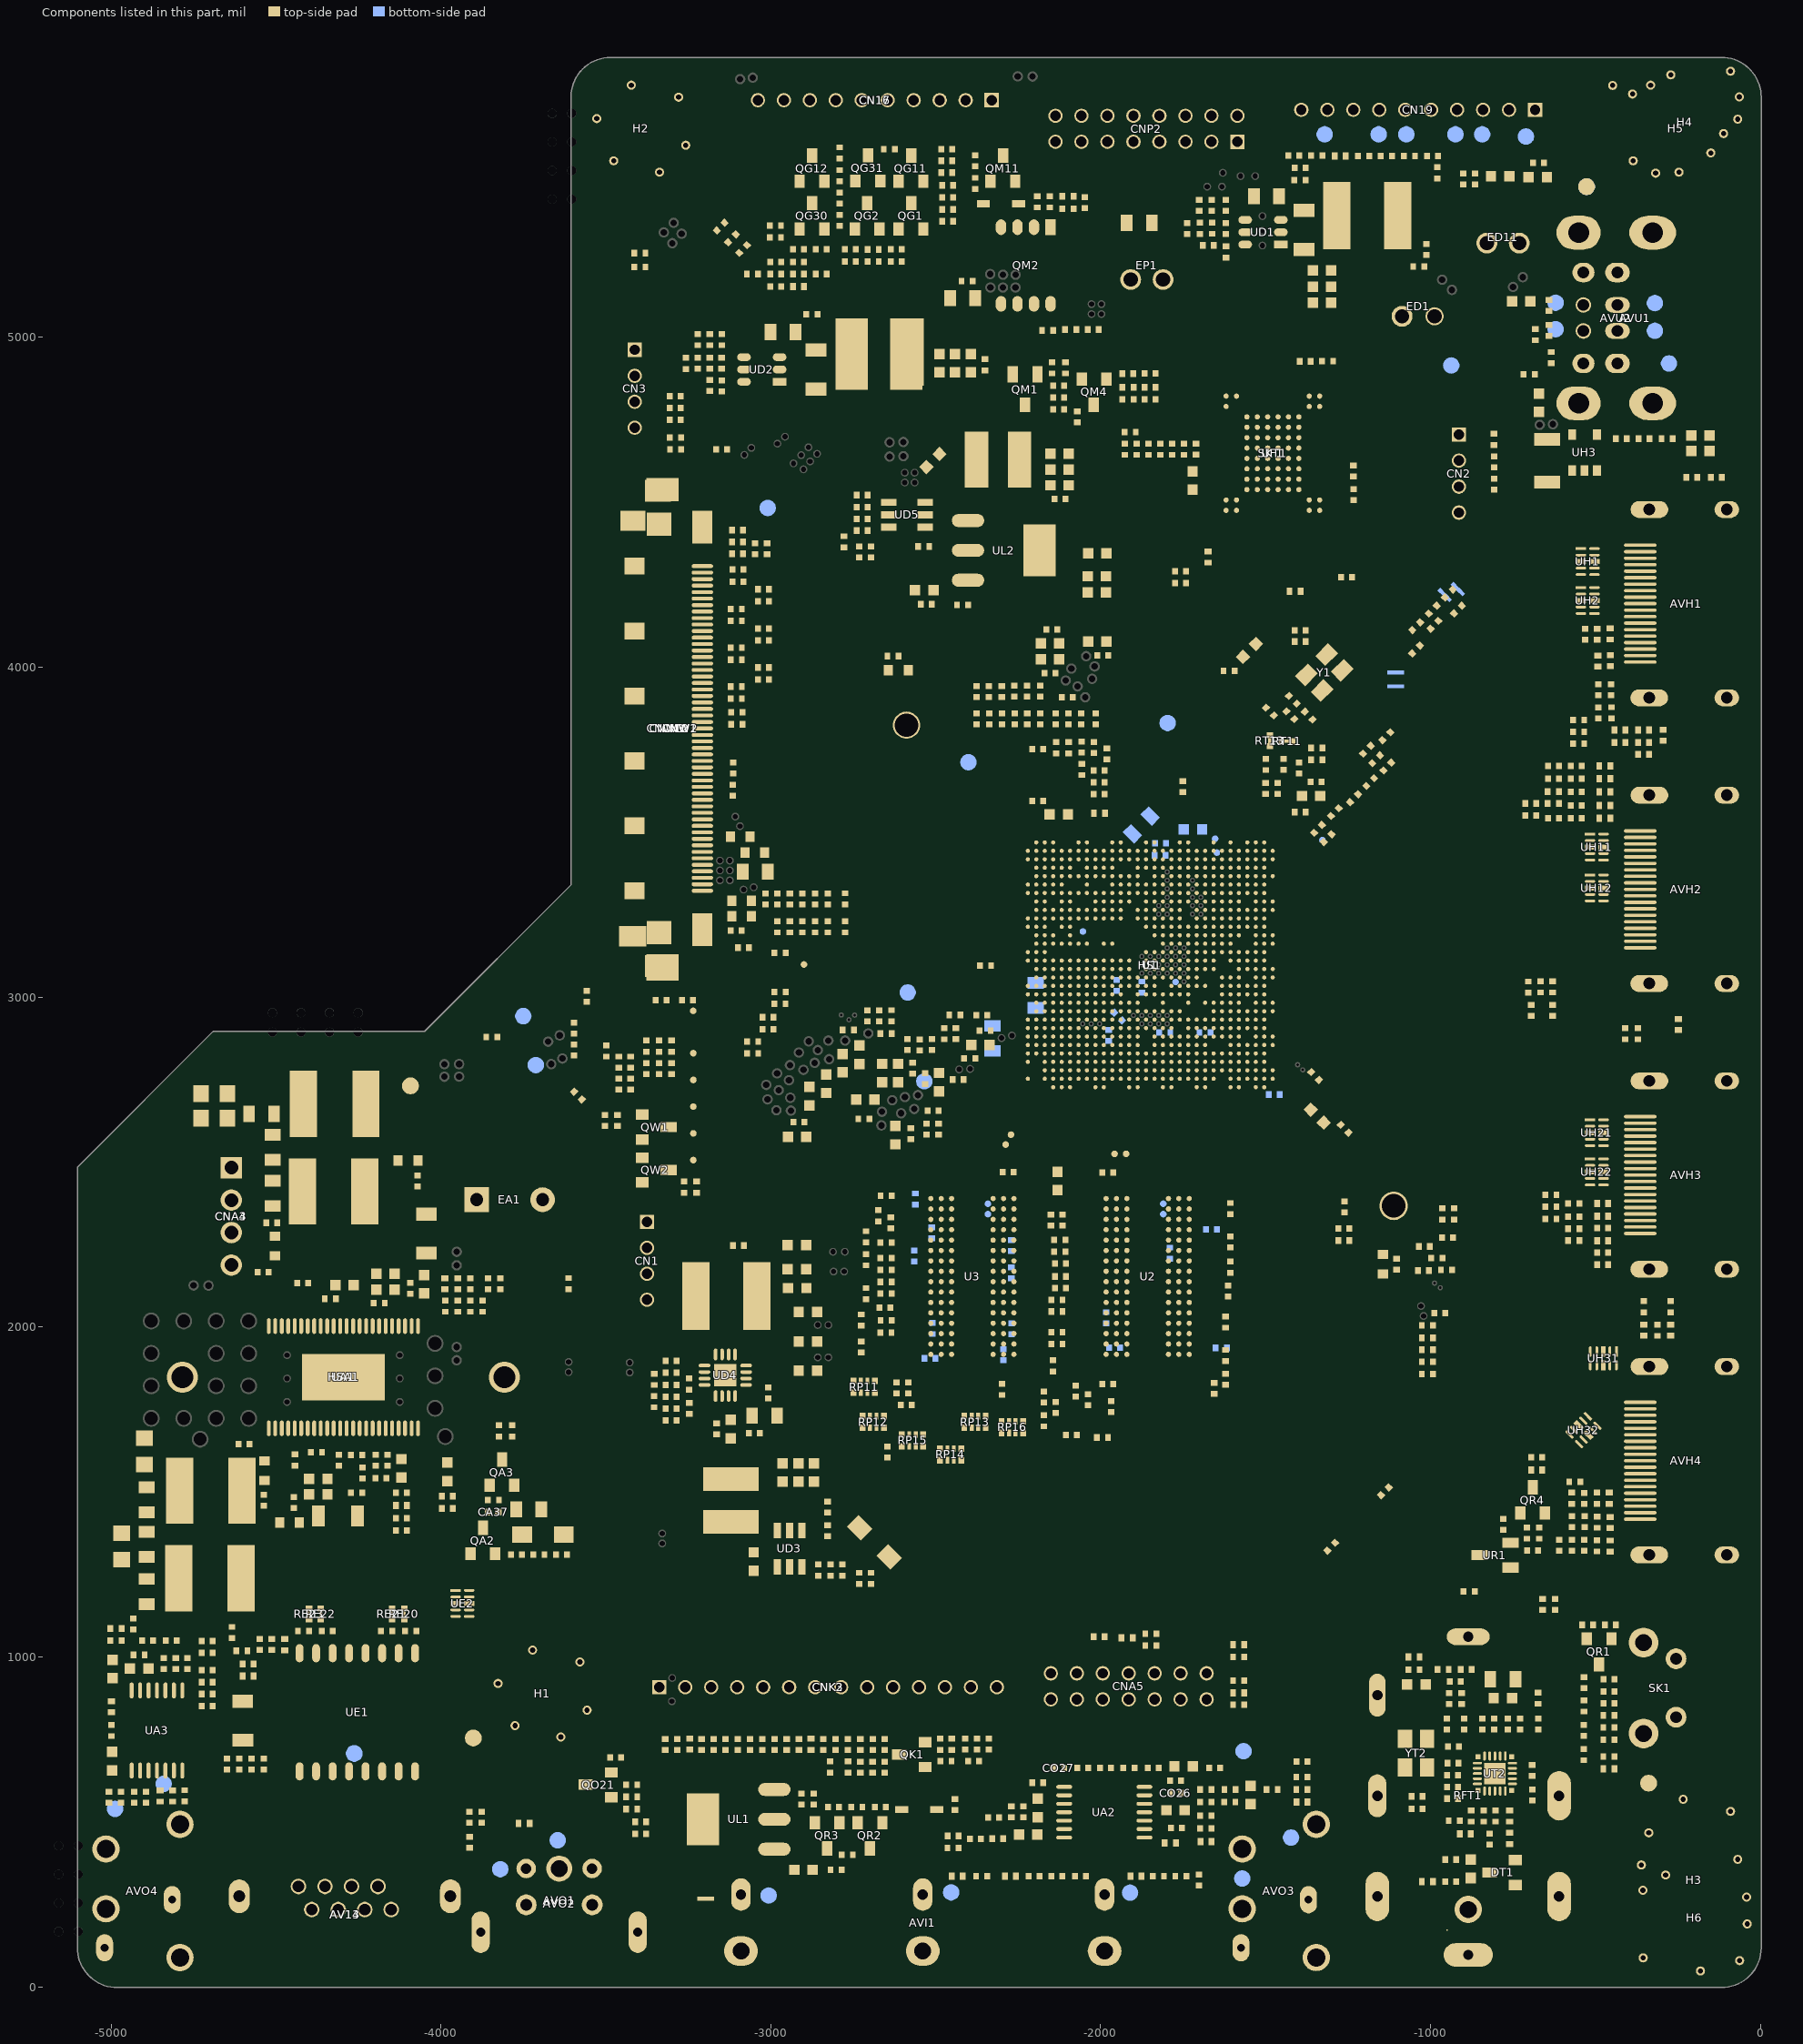
[diagram p0: the components of this part, seen from the top]
# Altium PCB MISC86290.PcbDoc (part 30 of 31)
Units mil, origin at the board's own origin, x right, y up, seen from the top; angles counter-clockwise.
Board outline 5104.71 x 5851.49 mil, 2 copper layers (TopLayer, BottomLayer), stack 61.855 mil thick; 1026 components, 667 nets, 4280 pads, 2294 vias.

## Other copper (continued)
BottomLayer:
  rectangle net GND: -1714.23,3506 -1676.5,3598.5
  rectangle net GND: -1723.5,2865.75 -1684.5,2918.16
  rectangle net GND: -3929.45,78 -3834,254.33
  rectangle net GND: -3978,211 -3889,336.95
  rectangle net GND: -4668,205 -4612.21,335.6
  rectangle: 1509.88,1166.59 1640.08,1245.33
  rectangle net GND: -644,5205 -158,5383.07
  rectangle net GND: -999.5,45.5 -767.5,160
  rectangle net GND: -1236.5,176.5 -1095.5,377
  rectangle net GND: -685,476 -533,705.5
  rectangle net GND: -1723.5,2918.16 -1658.13,2982
  rectangle net GND: -369.5,5302.5 -225,5406
  region net AVDD_EAR33/AU33: -1379.69,2771.69 -1370.69,2771.69 -1354.1,2755.1 -1354.1,2741.08 -1365.08,2741.08 -1372.94,2748.94 -1372.94,2764.94
  pour cut-out: -2568.5,693.5 -2536.5,693.5 -2529,701 -2521,701 -2521,683 -2504.5,666.5 -2533.6,637.4 -2546.39,637.4
  pour cut-out: -3287.55,3022.65 -3287.55,2990.74 -3270.17,2973.36 -3287,2956.53 -3287,2849 -3416,2849 -3418.88,2846.12 -3418.88,2983.69 -3387.76,3014.8
  pour cut-out: -952.79,1738.01 -1001.99,1738.01 -1001.66,1738.34 -1001.66,1760.19 -985.35,1776.5 -961.32,1776.5
  pour cut-out: -3092,3573.24 -3131.74,3573.24 -3146.5,3588 -3154,3580.5 -3159.5,3580.5 -3159.5,3538.5 -3128.14,3507.14 -3120,3507.14
  region net 3V3_M: -2004.5,3945 -2031,3945 -2060,3974 -2060,4044 -2054.5,4049.5 -2017.5,4049.5 -2001.5,4033.5 -2001.5,3992.5 -1985,3976 -1985,3965
  pour cut-out: -4598.5,226 -4598.5,185 -4593.5,180 -4551.5,180 -4549,182.5 -4549,239.5 -4550.5,241 -4584,241 -4597.5,227.5
  pour cut-out: -1678.84,1557.5 -1687.65,1566.3 -1687.65,1573 -1672.35,1573 -1670.34,1571 -1672.84,1568.5 -1672.84,1556.64
  region net NetCN2_4: 213 vertices and 0 holes, not listed, extent -934.4,4394.99 -893.6,4468.89
  region: -4442,180.67 -4442,62.56 -4134,62.56 -4134,180.67
  pour cut-out: -294.25,5156.5 -258.25,5120.5 -258.25,4895.5 -288.25,4865.5 -438.25,4865.5 -470.25,4897.5 -470.25,5119.5 -433.25,5156.5
  region net VCC_PANEL: -2376.26,5172.74 -2338.26,5210.74 -2253.26,5210.74 -2240.26,5197.74 -2240.26,5142.74 -2299.26,5083.74 -2376.26,5083.74
  region net 5V_M: -681,4778 -689,4770 -689,4721 -680,4712 -621,4712 -611.74,4721.26 -611.74,4741.74 -648,4778
  region net 3V3_M: -1759.52,3323.09 -1759.52,3264.26 -1738.02,3242.76 -1692.2,3242.76 -1687.02,3247.94 -1687.02,3279.26 -1691.23,3279.26 -1722.02,3310.05
  region net 5V_M: -3621,1911 -3459,1911 -3410.5,1862.5 -3421,1852 -3619,1852 -3625,1858 -3625,1907
  region net 0.95V_VDDC: -2759,2888 -2896,2888 -3053,2731 -3053,2710 -3039,2696 -2877,2696 -2761.25,2811.75 -2761.25,2883.53 -2757.93,2886.84
  region net 0.95V_VDDC: -3053,2731 -3053,2695 -2977,2619 -2921,2619 -2836,2704 -2836,2788 -2996,2788
  region net 5V_M: -3461,1911 -3422.5,1911 -3410.5,1899 -3410.5,1862 -3420.5,1852 -3456.5,1852 -3467.5,1863 -3467.5,1904.5
  pour cut-out: -1775.16,2878.47 -1836.34,2878.47 -1836.34,2878.46 -1836.34,2890.97 -1834,2893.31 -1775.16,2893.31
  region net GND: -2501.72,1910.03 -2469.72,1910.03 -2469.72,1854.03 -2485.72,1838.03 -2501.72,1838.03 -2501.72,1910.03
  region net GND: -2061.72,2046.03 -2061.72,2078.03 -1973.72,2078.03 -1973.72,2046.03 -2061.72,2046.03
  region net GND: -2341.72,1874.03 -2341.72,1906.03 -2253.72,1906.03 -2253.72,1874.03 -2341.72,1874.03
  region net GND: -2545.72,1954.03 -2545.72,1986.03 -2457.72,1986.03 -2457.72,1954.03 -2545.72,1954.03
  region net GND: -1905.72,1922.03 -1945.72,1922.03 -1945.72,1998.03 -1905.72,1998.03 -1905.72,1922.03
  region net GND: -2313.72,2206.03 -2313.72,2238.03 -2225.72,2238.03 -2225.72,2206.03 -2313.72,2206.03
  region net GND: -1601.72,1898.03 -1621.72,1898.03 -1621.72,1974.03 -1601.72,1974.03 -1601.72,1898.03
  region net GND: -1613.72,2262.03 -1653.72,2262.03 -1653.72,2338.03 -1613.72,2338.03 -1613.72,2262.03
  region net GND: -2581.72,2170.03 -2581.72,2202.03 -2525.72,2202.03 -2509.72,2186.03 -2509.72,2170.03 -2581.72,2170.03
  region net 1V5_DDR: -2476,2787 -2560.25,2787 -2654,2693.25 -2654,2677 -2647,2670 -2621,2670 -2607,2684 -2547,2684 -2476,2755
  region net LINEOUT_LL: -5024.75,458.5 -4945,458.5 -4940,453.5 -4940,380.5 -4944,376.5 -5023,376.5 -5033,386.5 -5033,450.25
  region net LINEOUT_LL: -5024.75,277.4 -4945,277.4 -4940,272.4 -4940,199.4 -4944,195.4 -5023,195.4 -5033,205.4 -5033,269.15
  region net GND: -5020,159 -4951,159 -4947,155 -4947,81 -4951,77 -5017,77 -5026,86 -5026,153
  pour cut-out: -5106,522 -4951.93,522 -4936.93,507 -4936.93,466.57 -4945,458.5 -5114.5,458.5 -5128,472 -5128,500
  pour cut-out: -4928,389 -4941,402 -5033,402 -5105,330 -5105,172.65 -5099.68,167.32 -4954.77,167.32 -4928,194.09
  pour cut-out: -3984,228 -3984,190 -3992,182 -4025,182 -4041,198 -4041,229 -4032,238 -3994,238
  pour cut-out: -516,5184 -381.61,5184 -368.01,5170.4 -368.01,5167.99 -376,5160 -525,5160 -525,5175
  region net CNW12_PIN42: -3117,3561 -3120,3558 -3120,3456.29 -3090,3426.29 -3090,3340.5 -3097,3333.5 -3097,3320.5 -3089,3312.5 -3049.5,3312.5 -3039,3323 -3039,3433.5 -3075,3469.5 -3075,3544 -3092,3561
  region net NetCN3_4: 213 vertices and 0 holes, not listed, extent -3432.9,4652.5 -3392.1,4726.39
  region net NetCN1_4: 213 vertices and 0 holes, not listed, extent -3395.65,2008.62 -3354.85,2082.52
  region net GND: -950.5,1113 -829,1113 -797.5,1081.5 -797.5,1034.5 -823,1009 -963,1009 -990,1036 -990,1110 -979.5,1120.5
  region net GND: -1178.5,674.5 -1127.5,674.5 -1103.5,650.5 -1103.5,505 -1120.5,488 -1189,488 -1227.5,526.5 -1227.5,631 -1197,661.5 -1197,679
  region net GND: -591.5,372 -638.5,372 -668.5,342 -668.5,211.5 -633,176 -599.5,176 -574,201.5 -574,231 -562.5,242.5 -562.5,372 -577.5,387
  region net GND: -1169,782 -1208,821 -1208,958 -1193,973 -1125,973 -1105,953 -1105,844 -1154,795 -1161.5,795 -1163,793.5
  region net GND: -1855.16,3030.54 -1969.76,3030.54 -1980.54,3019.77 -1979.36,3019.77 -1942.09,2982.5 -1863.57,2982.5 -1847.07,2999 -1815.5,2999
  region net GND: -1870.5,3437 -1870.5,3461.72 -1944.28,3535.5 -1963.61,3535.5 -1976,3523.11 -1976,3495 -1908,3427 -1867.5,3427
  pour cut-out: -3171.5,4711.5 -3171.5,4721.18 -3242.09,4791.77 -3429.05,4791.77 -3442.41,4805.13 -3442.41,4705.26 -3394.64,4657.5 -3356,4657.5
  pour cut-out: -3223.25,4579.25 -3223.25,4637.28 -3193.73,4666.8 -3207,4680.07 -3207,4689.5 -3304,4689.5 -3337.84,4655.66 -3337.84,4626.98
  region net GND: -285.8,4867.95 -288.25,4865.5 -576.77,4865.5 -613.77,4902.5 -624,4902.5 -609,4887.5 -609,4850.98 -618.84,4841.15 -597,4819.31 -597,4745.42 -597.39,4745.03 -588.5,4736.14 -588.5,4730 -546.5,4730 -542.5,4726 -500,4726 -453,4773 -425,4773 -354.5,4702.5 -226.5,4702.5 -184,4745 -184,4863 -165.5,4881.5
  pour cut-out: -578.5,4888 -668,4977.5 -668,5127 -649,5146 -623,5146 -596,5173 -562,5173 -502.5,5113.5 -502.5,5027
  region net GND: -3369,942.5 -3373,946.5 -3396,946.5 -3400.5,951 -3400.5,952 -3384,952 -3373,963 -3369,963
  pour cut-out: -3492,638.5 -3380,638.5 -3359.5,618 -3338,639.5 -3318,639.5 -3318,683.62 -3346.87,654.75 -3486,654.75
  region net 1V5_DDR: -2537.5,2697 -2537.5,2657 -2602,2592.5 -2680,2592.5 -2686.5,2599 -2686.5,2660.75 -2590.75,2756.5 -2525,2756.5 -2522.5,2759
  region net 3V3_STB: -1428.16,2740.51 -1225.5,2537.85 -1225.5,2476.54 -1428.91,2679.95 -1428.91,2740.51
  region net GND: -1610.5,2899 -1539.34,2899 -1530.32,2889.98 -1611.22,2889.98 -1616.84,2895.6 -1616.84,2896.14
  region net 0.95V_VDDC: -2014.5,3136 -2041,3109.5 -2358.5,3109.5 -2375.5,3092.5 -2375.5,3041 -2354,3019.5 -1993.5,3019.5 -1971.5,3041.5 -1971.5,3136
  region net 3V3_STB: -1666.96,2902.49 -1638.89,2902.49 -1620.18,2883.78 -1533.19,2883.78 -1518.51,2869.1 -1518.51,2859.11 -1522.42,2855.2 -1567.1,2855.2 -1579.1,2867.2 -1628.52,2867.2 -1644.02,2882.7 -1658.94,2882.7 -1667.19,2890.95 -1667.19,2901.92
  region net GND: -1389,2747.81 -1389,2760.81 -1427.9,2799.71 -1427.9,2801.7 -1524.73,2898.53 -1536.16,2898.53 -1536.16,2897.34 -1406.32,2767.5 -1406.32,2753.9 -1398.15,2745.73 -1396.91,2745.73
  pour cut-out: -702.64,3166.16 -702.64,3161.48 ccw(c-682.52,3161.48) -696.75,3147.25 ccw(c-681,3163) -681,3140.73 -570.9,3140.73 ccw(c-570.9,3151.9) -563,3144 cw(c-535.62,3171.38) -574.34,3171.38 -574.34,3197 cw(c-574.34,3233.59) -600.22,3207.72 -612.5,3220 ccw(c-636.26,3196.24) -636.26,3229.84 -666.84,3229.84
  text ".GBL" at 2085.1,1188.26 h60
  text "BottomLayer" at 1662.68,1186.76 h60

## Silkscreen, mask and mechanical layers (free items; w line width, h text height)
TopOverlay:
  drawing of 267 lines, arcs and shapes, not listed
  text "Solder Mask:" at 1375,6344.9 h60
  text "IPC SM-840" at 1787.5,6343.9 h60
  text "Silkscreen Color:" at 2553.5,6343.9 h60
  text "White" at 3032.5,6343.9 h60
  text "Units:" at 2553.5,6244.9 h60
  text "PTH Copper Thickness:" at 1375,6243.9 h60
  text ">20um" at 2048.5,6242.9 h60
  text "mm" at 2751.5,6243.4 h60
  text "Dielectric Constant Er@1GHz To 1MHz:" at 1374.66,6144.92 h60
  text "4.2 --- 4.6" at 2554.16,6145.42 h60
  text "Panel Size:" at 1373,6046.4 h60
  text "2L,2,111.28×148.50mm,FR4(TG150-CTI175),1OZ,Green,OSP,1.2mm" at 1678.16,6046.42 h60
  text "Silkscreen on PTH:" at 1373.5,5944.9 h60
  text "Primary Side Retained;" at 1891.5,5943.9 h60
  text "Secondary Side  Removed for Soldering" at 2553.5,5942.4 h60
  text "Special Requirements" at 1372.49,5854.21 h60
  text "For engineering questions with no reply within 2 hours, call: PHONE_A" at 3259.16,5846.92 h60
  text "POWER" at -2125,5789.5 h60
  text "EXT-WIFI" at -1017,5788 h60
  text "2" at -6473.13,5777.09 h160 r180
  text "1. Lead-free HASL (HAL_LF, Lead Free Hot Air Leveling)" at 1963.38,5750.63 h60
  text "2. Organic solderability preservative (OSP, Organic Solderability Preservatives)" at 1963.38,5666.63 h60
  text "3. Electroless nickel immersion gold (ENIG, Electroless Nickel/Immersion Gold)" at 1961.88,5575.13 h60
  text "Plated Technics" at 1447.5,5540.4 h60
  text "4. Electroless nickel immersion gold + gold finger (ENIG_G/F, Electroless Nickel/Immersion Gold + Gold Finger)" at 1963.38,5494.63 h60
  text "5. Gold plating (Gold_plated, Gold-plated)" at 1964.38,5414.13 h60
  text "LOCAL DIMMING" at -3148,5389 h60 r90
  text "6. Gold plating + gold finger (Gold_Plated_G/F, Gold-plated + Gold Finger)" at 1964.88,5336.13 h60
  text "PM-UART" at -3565,5118.5 h60
  text "Impedance Control" at 1377.24,5107.54 h60
  text "Target Impedance" at 2174.07,5107.64 h60
  text "Width & Clearance" at 2919.9,5107.41 h60
  text "Layer(s)" at 3688.21,5107.72 h60
  text "75 +/- 10% Ohm" at 2196.27,5006.94 h60
  text "G/12/15.8/12/G mil" at 2877.32,5006.26 h60
  text "layer 1" at 3688.21,5006.38 h60
  text "Single End Impedance" at 1377.24,4960.72 h60
  text "DEBUG" at -1025,4865 h60
  text "[ Zo ]" at 1600.74,4823.47 h60
  text "G/5/7/5/7/5/G mil" at 2887.32,4615.26 h60
  text "100 +/- 10% Ohm" at 2183.27,4614.25 h60
  text "layer 1" at 3704.5,4612.5 h60
  text "Differential Impedance" at 1377.1,4559.14 h60
  text "[ Zo ]" at 1600.23,4435.8 h60
  text "( G: Ground )" at 1510.31,4328.3 h60
  text "90 +/- 10% Ohm" at 2209.32,4316.26 h60
  text "G/5/11/5/11/5/G mil" at 2887.32,4312.76 h60
  text "layer 1&2" at 3703.5,4307.5 h60
  text "Common Mode Impedance" at 1356.87,4106.62 h60
  text "[ Zc ]" at 1604.87,4025.62 h60
  text "Refer to Gerber documents GTP&GBP for Stencil aperture design" at 2271.93,3761.43 h60
  text "[Bottom-side parts: stencil per BOM]" at 2271.2,3674.01 h60
  text "Stencil" at 1371.16,3664.42 h60
  text "New" at 2269.83,3566.88 h60
  text "V_by_one" at -3017,3549 h60 r90
  text "Test fixture (Testing jig)" at 1369.25,3468.78 h60
  text "The same as XXXXXXXXXXX XXXXXX" at 2258,3468.5 h60
  text "The same as XXXXXXXXXXX XXXXXX" at 2258.5,3375.5 h60
  text "Wave-soldering fixture (Wave-soldering jig)" at 1371.47,3370.54 h60
  text "Solder paste" at 2269.45,3268.76 h60
  text "Production process" at 1369.95,3267.26 h60
  text "[Process and notes]" at 1550.16,3182.42 h60
  text "Back-side panelization" at 2267.22,3069.97 h60
  text "Special requirements (Special Requirements)" at 1370.95,3069.26 h60
  text "Chip parts on solder side taller than 2mm (wave soldering)" at 1370.66,2967.92 h60
  text "Packaging notes (Package Attention)" at 1370.33,2871.71 h60
  text "[Easily damaged parts]" at 1611.66,2786.92 h60
  text "New footprint matching (Footprint Matching)" at 1370.33,2671.71 h60
  text "[New component footprint]" at 1597.66,2587.92 h60
  text "(Automated Testing Support)" at 1688.66,2473.42 h45
  text "Automatic test support" at 1370.16,2469.92 h60
  text "[Reserved vacuum nozzle and press-pin positions]" at 1530.66,2385.42 h60
  text "Layer Stack Up Detail for" at 1511.26,2025.89 h100
  text ".Pcb_File_Name_No_Path" at 2572.08,2025.89 h100
  text "FRC PLACE HOLDER" at -3520.75,1975 h60 r90
  text "Layer" at 1675.62,1878.17 h50
  text "Gerber" at 2047.34,1878.17 h50
  text "Layer" at 2358.49,1878.17 h50
  text "Layer" at 2994.72,1878.17 h50
  text "Copper" at 3783.63,1878.17 h50
  text "Dielectric" at 4095.41,1878.17 h50
  text "Height" at 4095.5,1833 h50
  text "Stack up" at 2992,1832 h50
  text "Name" at 1675.62,1825.79 h50
  text "Document" at 2047.34,1825.79 h50
  text "Ordor" at 2358.49,1825.79 h50
  text "Thickness" at 3783.63,1825.79 h50
  text "SPEAKER" at -4982,1714 h60 r90
  text "TopOverlay" at 1675.33,1592.93 h60
  text ".GTO" at 2084.9,1590.37 h60
  text "0.4mil" at 4092.72,1505.34 h60
  text "1" at 2411.69,1402.19 h60
  text "1.4mil" at 3796.68,1402.13 h60
  text "2" at 2411.74,1189.15 h60
  text "1.4mil" at 3794.97,1188.14 h60
  text "ATMOS AND DEBUG" at -2166,1146 h60
  text "0.4mil" at 4095.4,1093.46 h60
  text "Notes:" at 1347.19,530.59 h80
  text "1. No Plated Through Hole  overlap each other should be combined ,Residues between them should be eliminated." at 1346.32,442.68 h60
  text "2. Plated Through Hole superposition should be made as a bigger one." at 1346.26,366.58 h60
  text "3. When there is not enough space for UL authentication marking,Manufacturer ID code and the Bar Code frame," at 1346.32,298.08 h60
  text "only the Manufacturer  ID code is needed and layed wherever it can be." at 1404.7,227.39 h60
  text "4. Spacing between two pads of IC package should be covered with solder oil." at 1346.32,150.62 h60
  text "5. All trace should be covered with green oil unless otherwise specified. If discovers unusually, please confirm with us." at 1346.32,77.21 h60
  text "1" at -2289.22,69.37 h160
  text "6. Silkscreen overlaped SMD pads should be removed directly." at 1346.32,3.9 h60
  text "7. The width of Carbon Sprayed must be 16mil wider than its trace." at 1346.32,-67.14 h60
  text "8. Bridging Thickness of V-cut  should be kept within 0.3±0.1mm when the width of single piece bare board is smaller than 20mm." at 1346.32,-141.57 h60
  text "9. There is no need to plugged with green oil when the diameter of vias is bigger than 0.6mm." at 1346.32,-223.4 h60
  text "10. All vias under BGA must be covered and plugged with Solder oil." at 1346.33,-303.27 h60
BottomOverlay:
  rectangle: 1509.88,974.82 1640.08,1053.56
  region: -400,2670 -400,2694.1 -425.9,2720 -485,2720 -500,2705 -500,2215 -443,2215 -443,2627
  region: -435,3160 -493,3160 -493,3520 -435,3520
  region: -440,3315 -440,3275 -420,3255 -420,3213.5 -437.25,3196.25 -450,3209 -450,3305
  region: 16 vertices and 3 holes, not listed, extent -3400.9,113.96 -3115.45,536.16
  lines w5: -4669,2530 -4867,2530 -4867,2143 -4665,2143 ; -3441.5,4690 -3565.5,4690 -3565.5,4996 -3435.5,4996 ; -3399,2355 -3644,2355 -3644,2046 -3398,2046 ; -3385,912 -3385,1107.61 -2264,1107.61 -2264,907.34 ; -2193,975.73 -2193,1297 -1632,1297 -1632,967 ; -1534,5549 -1505,5520 -1501,5520 -1343,5520 -1343,5475 ; -1430,5710 -1430,5832 -646,5832 -646,5717 ; -1359,5491 -1343,5475 ; -1327,5491 -1343,5475 ; -933,4433 -1102,4433 -1102,4743 -933,4743 ; 2060.78,974.82 2060.78,1053.56 ; -1365.48,5202.5 -926,5202.5 -926,5475 -1335,5475 -1365.48,5475 -1365.48,5202.5 ; -1206.92,1240.13 -773.85,1240.13 -773.85,1692.89 -1206.92,1692.89 -1206.92,1240.13 ; 1509.88,974.82 2241.92,974.82 2241.92,1053.56 1509.88,1053.56 1509.88,974.82
  text "MISO" at -2429.5,5806.5 h50
  text "EN" at -2307,5806 h50
  text "GND" at -2920,5805 h50
  text "HSY" at -2764,5805 h50
  text "GND" at -2591.5,5805.5 h50
  text "GND" at -1307,5785 h60
  text "GND" at -1167,5784 h60
  text "3V3" at -723,5784.5 h60
  text "WAKE" at -986,5783 h60
  text "DP" at -884,5782 h60
  text "LD" at -2855.5,5767.5 h50
  text "CLK" at -2514.5,5767 h50
  text "CSN" at -2965,5766 h50
  text "CSZ" at -2356,5766.5 h50
  text "VSY" at -2681.5,5765.5 h50
  text "REG" at -1112,5737 h60
  text "GND" at -941,5737 h60
  text "DM" at -811,5737 h60
  text "3V3" at -657.5,5737.5 h60
  text "HOST" at -1241,5736 h60
  text "12V" at -1103,5371 h50 r270
  text "GND" at -1063,5371 h50 r270
  text "12V" at -1147,5370 h50 r270
  text "VCC" at -1021,5370 h50 r270
  text "ADJ" at -1321,5369 h50 r270
  text "DIM" at -1278,5369 h50 r270
  text "GND" at -1234,5369 h50 r270
  text "GND" at -1191,5369 h50 r270
  text "GND" at -1191,5264 h50 r270
  text "GND" at -1233,5263 h50 r270
  text "12V" at -1147,5263 h50 r270
  text "GND" at -1063,5263 h50 r270
  text "BLO" at -1319,5262 h50 r270
  text "PWN" at -1277,5262 h50 r270
  text "12V" at -1102,5262 h50 r270
  text "VCC" at -1020,5261 h50 r270
  text "POWER&INVERTER" at -934,5213 h50
  text "USB IN" at -66.15,4947.64 h60 r270
  text "3V3" at -3464.25,4940.75 h50
  text "GND" at -3460,4864.5 h50
  text "RX2" at -3464.25,4783.27 h50
  text "TX2" at -3464.25,4704.53 h50
  text "3V3" at -968,4684.28 h60
  text "GND" at -971,4594.68 h60
  text "HDMI 4(2.0) (ARC)IN" at -46,4545 h60
  text "SCL" at -978,4517.68 h60
  text "SDA" at -975.5,4446.5 h60
  text "HDMI 3 IN(2.0)" at -555,3150 h60 r270
  text "HDMI 2 IN(2.0)" at -38,2828 h60
  text "ROUT+" at -4703,2473 h50
  text "ROUT-" at -4703,2373 h50
  text "TX1" at -3424,2300.74 h60
  text "LOUT-" at -4703,2278 h50
  text "RESETN" at -3424,2222 h60
  text "LOUT+" at -4703,2173 h50
  text "ALIVE" at -3424,2143.26 h60
  text "RCR" at -3424,2064.52 h60
  text "HDMI 1 IN(2.0)(UART)" at -34,1947 h60
  text "SCL" at -2171,1140 h60 r270
  text "GND" at -2092.26,1140 h60 r270
  text "MUTE" at -2013.52,1140 h60 r270
  text "3V3" at -1934.78,1140 h60 r270
  text "SD1" at -1856.04,1140 h60 r270
  text "SD" at -1777.3,1140 h60 r270
  text "MCK" at -1698.56,1140 h60 r270
  text "SDA" at -2171,1013 h60 r270
  text "GND" at -2092.26,1013 h60 r270
  text "RST" at -2013.52,1013 h60 r270
  text "3V3" at -1934.78,1013 h60 r270
  text "SD2" at -1856.04,1013 h60 r270
  text "WS" at -1777.3,1013 h60 r270
  text "BCK" at -1698.56,1013 h60 r270
  text ".GBO" at 2085.51,997.85 h60
  text "BottomOverlay" at 1663.84,996.86 h60
  text "Reset" at -77,899 h60
  text "RF IN" at -673,186 h60
  text "LINE OUT" at -4912,62.5 h60 r270
  text "COAX OUT" at -3493,58 h60
  text "AV INT" at -2274,30 h60
  text "RJ45 IN" at -4201,16 h60
  text "HEADPHONE OUT" at -1400,14 h60
  text "OPTICAL OUT" at -3453,12 h60
TopPaste:
  rectangle: 1509.88,1668.23 1640.08,1746.97
  lines w5: 2060.78,1668.23 2060.78,1746.97 ; 1509.88,1668.23 1509.88,1746.97 2241.92,1746.97 2241.92,1668.23 1509.88,1668.23
  text "TopPaste" at 1675.33,1689.46 h60
  text ".GTP" at 2084.9,1687.33 h60
BottomPaste:
  rectangle: 1509.88,880.67 1640.08,959.41
  lines w5: 2060.78,880.67 2060.78,959.41 ; 1509.88,880.67 1509.88,959.41 2241.92,959.41 2241.92,880.67 1509.88,880.67
  text "BottomPaste" at 1662.68,903.65 h60
  text ".GBP" at 2085.78,898.53 h60
TopSolder:
  rectangle: 1509.88,1478.28 1640.08,1557.02
  lines w5: 2060.78,1478.28 2060.78,1557.02 ; 1509.88,1478.28 1509.88,1557.02 2241.92,1557.02 2241.92,1478.28 1509.88,1478.28
  text "TopSolder" at 1675.83,1498.38 h60
  text ".GTS" at 2084.9,1496.73 h60
BottomSolder:
  drawing of 50 lines, arcs and shapes, not listed
  text "BottomSolder" at 1662.68,1090.06 h60
  text ".GBS" at 2084.86,1089.17 h60
过炉治具:
  drawing of 232 lines, arcs and shapes, not listed
3D和装配:
  circle w2.5: c444.93,3607.26 r1.25
  circle w2.5: c1115.74,905.51 r1.25
  circle w2.5: c1273.22,1594.49 r1.25
  circle w2.5: c1430.71,2460.63 r1.25
  circle w2.5: c-885.83,-966.64 r1.25
  circle w2.5: c-1968.51,-1124.12 r1.25
  circle w2.5: c649.6,3326.77 r1.25
  circle w2.5: c649.6,4192.92 r1.25
  circle w2.5: c649.6,4192.92 r1.25
  circle w2.5: c649.6,3326.77 r1.25
  circle w2.5: c-2421.38,1730.26 r1.25
  circle w2.5: c-2421.38,1730.26 r1.25
  circle w2.5: c-2303.27,1848.37 r1.25
  circle w2.5: c-2303.27,1848.37 r1.25
  circle w2.5: c-2303.27,1848.37 r1.25
  circle w2.5: c-2303.27,1848.37 r1.25
  circle w2.5: c-1968.51,-468.3 r1.25
  circle w2.5: c-2303.27,1848.37 r1.25
  circle w2.5: c-885.83,-84.64 r1.25
  circle w2.5: c-2303.27,1848.37 r1.25
  circle w2.5: c-314.05,-809.16 r1.25
  circle w2.5: c-314.05,-482.28 r1.25
  circle w2.5: c-2303.27,1848.37 r1.25
  circle w2.5: c373.01,-614.68 r1.25
  circle w2.5: c-2303.27,1848.37 r1.25
  circle w2.5: c-2421.38,1730.26 r1.25
  circle w2.5: c-2421.38,1730.26 r1.25
  circle w2.5: c-2421.38,1730.26 r1.25
  circle w2.5: c-2421.38,1730.26 r1.25
  circle w2.5: c-2421.38,1730.26 r1.25
  circle w2.5: c-2421.38,1730.26 r1.25
  circle w2.5: c-2421.38,1730.26 r1.25
  circle w2.5: c-1182.62,1402.87 r1.25
  circle w2.5: c-2421.38,1730.26 r1.25
  circle w2.5: c-2421.38,1730.26 r1.25
  circle w2.5: c-2073.35,1927.11 r1.25
  circle w2.5: c-2421.38,1730.26 r1.25
  circle w2.5: c-2501.37,1927.11 r1.25
  circle w2.5: c-2545.26,1839.02 r1.25
  circle w2.5: c-2457.47,2015.21 r1.25
  circle w2.5: c-3070.87,-1281.6 r1.25
  circle w2.5: c4239.32,6875.01 r1.25
  circle w2.5: c3844.99,6717.53 r1.25
  circle w2.5: c2860.74,6560.05 r1.25
  circle w2.5: c1588.19,3326.77 r1.25
  circle w2.5: c1745.67,4192.92 r1.25
  circle w2.5: c1903.15,5059.06 r1.25
  circle w2.5: c2060.63,5629.93 r1.25
  circle w2.5: c2218.11,5708.67 r1.25
  circle w2.5: c374.01,7329.46 r1.25
  circle w2.5: c275.59,7486.94 r1.25
  circle w2.5: c-2814.96,7644.42 r1.25
  circle w2.5: c-3114.18,7801.9 r1.25
  circle w2.5: c2411.36,5846.46 r1.25
  circle w2.5: c452.76,7086.62 r1.25
  circle w2.5: c2568.84,7086.62 r1.25
  circle w2.5: c-4105.3,1454.83 r1.25
  circle w2.5: c-3072.12,-307.09 r1.25
  circle w2.5: c-3721.1,-78.74 r1.25
  circle w2.5: c-4115.43,118.11 r1.25
  circle w2.5: c-3115.42,885.83 r1.25
  circle w2.5: c-3997.31,0 r1.25
  circle w2.5: c-3115.42,885.83 r1.25
  circle w2.5: c-3997.31,0 r1.25
  circle w5: c-3119,312.5 r984.25
  lines w5: -6865.38,-828.22 -6865.38,-946.33 -6747.27,-946.33 ; -5976,5629.92 240.5,5629.92
  lines w78.74: -4544,671 -4544,1052 ; -4514,809 -4646.5,809 -4704.5,751 -4704.5,635 -4653,583.5 -4248,583.5 ; -3962,627.5 -3962,1008.5
  text "2L,2,111.28×148.50mm,FR4(TG150-CTI175),1OZ,Green,OSP,1.2mm,4,64,90.4%,2979,0.2mm" at 1678.16,6046.42 h60
顶层限制:
  drawing of 3818 lines, arcs and shapes, not listed